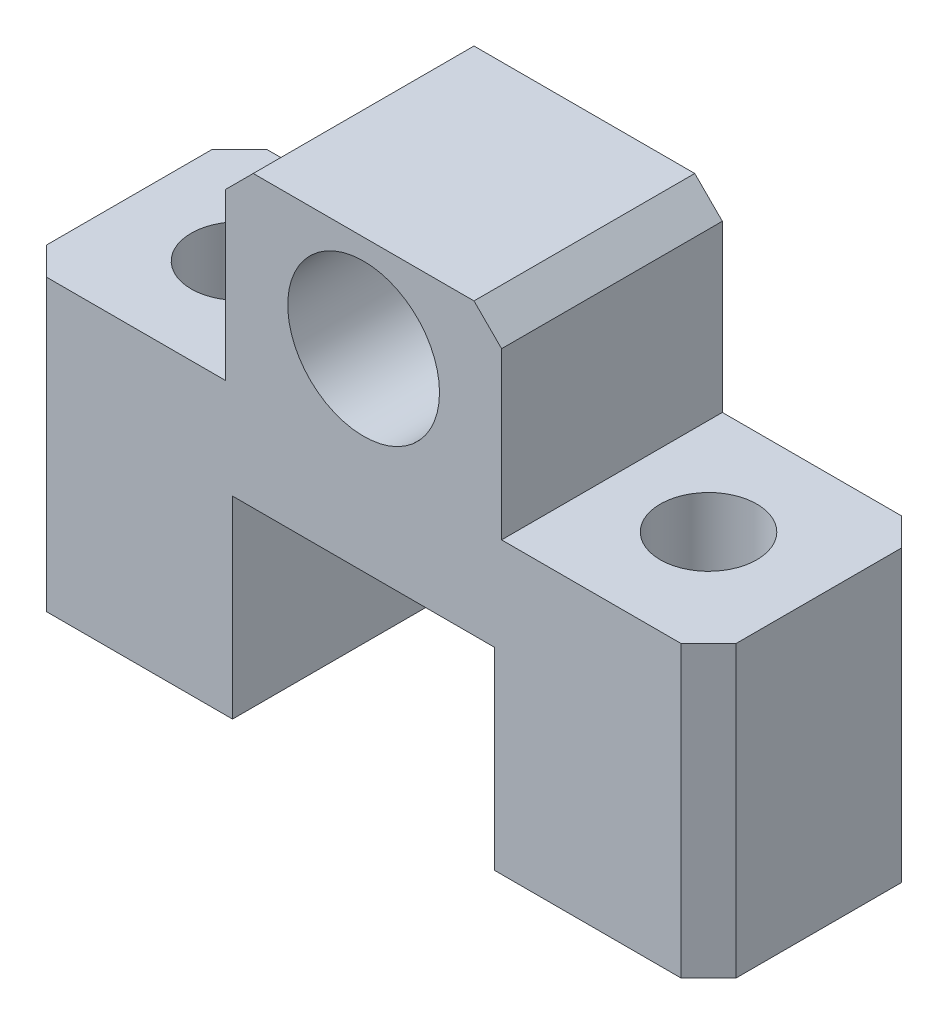
SolidWorks part; units mm, degrees
ref_plane "Front Plane" through (0, 0, 0) normal (0, 0, 1) x (1, 0, 0)
ref_plane "Top Plane" through (0, 0, 0) normal (0, 1, 0) x (1, 0, 0)
ref_plane "Right Plane" through (0, 0, 0) normal (1, 0, 0) x (0, 0, -1)
sketch "Sketch1" plane through (0, 0, 0) normal (0, 0, 1) x (1, 0, 0)
  line L1 (-12.5, -8.75) -> (12.5, -8.75)
  line L2 (-12.5, -8.75) -> (-12.5, 8.75)
  line L3 (-12.5, 8.75) -> (12.5, 8.75)
  line L4 (12.5, -8.75) -> (12.5, 8.75)
  line L5 (-12.5, -8.75) -> (12.5, 8.75) construction
  line L6 (-12.5, 8.75) -> (12.5, -8.75) construction
  point P0 (0, 0)
  dimension "D1" = 25
  dimension "D2" = 17.5
extrude "Boss-Extrude1" add sketch "Sketch1" along normal blind 8
sketch "Sketch2" plane through (0, 0, 8) normal (0, 0, 1) x (1, 0, 0)
  line L0 (0, 0) -> (0, 50000) construction
  line L1 (12.5, 8.75) -> (-12.5, 8.75) construction
  line L2 (12.5, 1.75) -> (5, 1.75)
  line L3 (-12.5, 8.75) -> (-5, 8.75)
  line L4 (-12.5, 8.75) -> (-12.5, 1.75)
  line L5 (-12.5, 1.75) -> (-5, 1.75)
  line L6 (-5, 8.75) -> (-5, 1.75)
  line L7 (5, 8.75) -> (5, 1.75)
  line L8 (12.5, 8.75) -> (5, 8.75)
  line L9 (12.5, 8.75) -> (12.5, 1.75)
  point P5 (0, 8.75)
  dimension "D1" = 7.5
  dimension "D2" = 7
extrude "Cut-Extrude1" cut sketch "Sketch2" against normal blind 8
sketch "Sketch3" plane through (0, 0, 8) normal (0, 0, 1) x (1, 0, 0)
  line L0 (-12.5, -8.75) -> (12.5, -8.75) construction
  line L1 (-4.75, -1.75) -> (4.75, -1.75)
  line L2 (-4.75, -1.75) -> (-4.75, -8.75)
  line L3 (-4.75, -8.75) -> (4.75, -8.75)
  line L4 (4.75, -1.75) -> (4.75, -8.75)
  line L5 (-4.75, -1.75) -> (4.75, -8.75) construction
  line L6 (-4.75, -8.75) -> (4.75, -1.75) construction
  point P0 (0, -5.25)
  dimension "D1" = 9.5
  dimension "D2" = 7
extrude "Cut-Extrude2" cut sketch "Sketch3" against normal through all
sketch "Sketch4" plane through (0, 0, 8) normal (0, 0, 1) x (1, 0, 0)
  line L0 (5, 8.75) -> (-5, 8.75) construction
  circle A0 centre (0, 5.25) radius 2.75
  dimension "D1" = 5.5
  dimension "D2" = 3.5
extrude "Cut-Extrude3" cut sketch "Sketch4" against normal blind 5
hole_wizard "Ø3.5 (3.5) Diameter Hole1" positions "Sketch5" profile "Sketch6" hole size "Ø3.5" standard "GB" end condition through all
sketch "Sketch5" plane through (0, 1.75, 0) normal (0, 1, 0) x (1, 0, 0)
  line L0 (-8.5, 0) -> (-8.5, -8) construction
  line L4 (0, 0) -> (0, -50000) construction
  line L5 (-12.5, -8) -> (-5, -8) construction
  line L6 (-12.5, 0) -> (-5, 0) construction
  point P0 (-8.5, -4)
  point P18 (8.5, -4)
  dimension "D1" = 17
sketch "Sketch6" plane through (-8.5, 1.75, 4) normal (1, 0, 0) x (0, 0, 1)
  line L0 (0, 0) -> (0, 10.5)
  line L1 (0, 10.5) -> (1.75, 10.5)
  line L2 (1.75, 10.5) -> (1.75, 0)
  line L5 (1.75, 0) -> (0, 0)
  line L11 (0, -6.35) -> (0, 107.95) construction
  dimension "通孔孔直径" = 3.5
  dimension "通孔孔深度" = 10.5
chamfer "Chamfer1" distance 1 angle 45 6 edges at (-5, 8.75, 4) (5, 8.75, 4) (12.5, -3.5, 0) (12.5, -3.5, 8) (-12.5, -3.5, 0) (-12.5, -3.5, 8)
